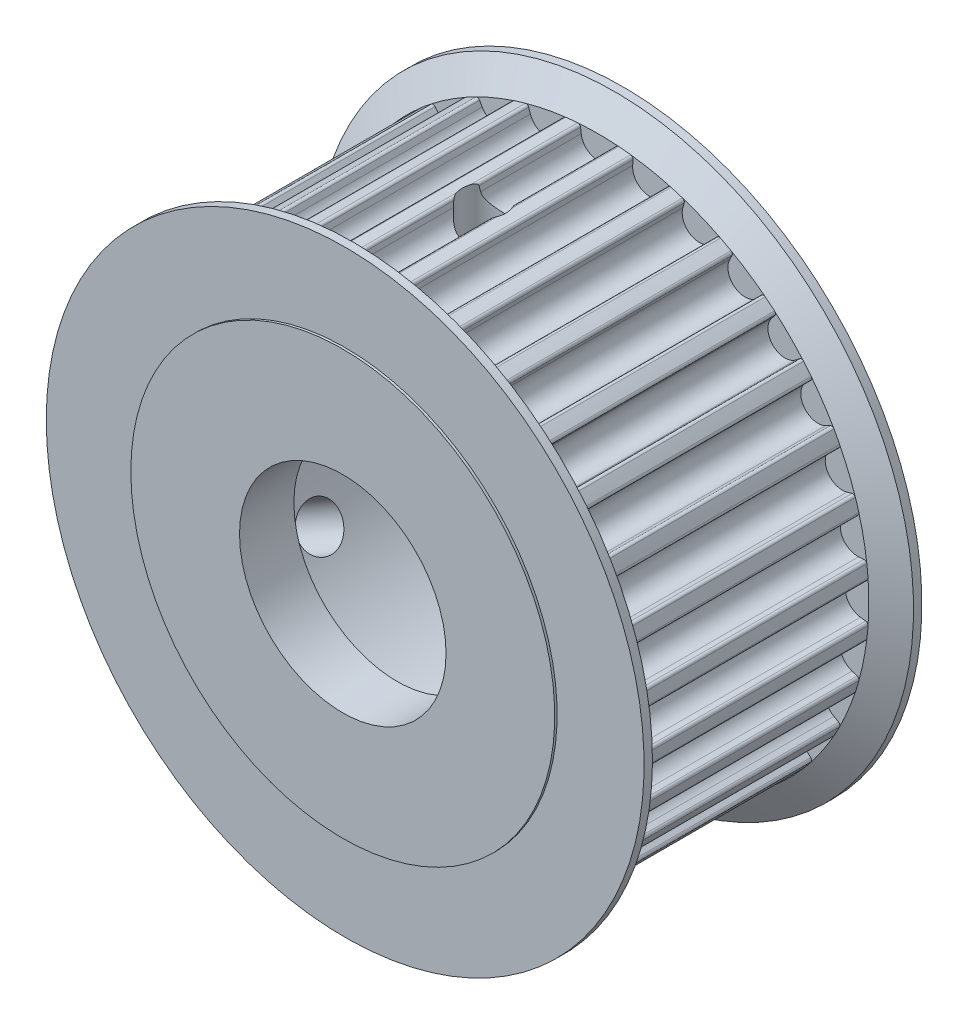
SolidWorks part; units mm, degrees
ref_plane "前视基准面" through (0, 0, 0) normal (0, 0, 1) x (1, 0, 0)
ref_plane "上视基准面" through (0, 0, 0) normal (0, 1, 0) x (1, 0, 0)
ref_plane "右视基准面" through (0, 0, 0) normal (1, 0, 0) x (0, 0, -1)
sketch "草图1" plane through (0, 0, 0) normal (1, 0, 0) x (0, 0, -1)
  line L0 (0, 0) -> (-26, 0) construction
  line L1 (0, 5) -> (-26, 5)
  line L2 (0, 5) -> (0, 19.5)
  line L4 (-0.22, 27.5) -> (-0.99, 27.5)
  line L5 (0, 19.5) -> (-0.22, 19.5)
  line L6 (-2.5, 24.895) -> (-23.5, 24.895)
  line L7 (-0.22, 19.5) -> (-0.22, 27.5)
  line L8 (-0.99, 27.5) -> (-2.5, 24.895)
  line L9 (-13, 0) -> (-13, 25.465) construction
  line L11 (-25.01, 27.5) -> (-23.5, 24.895)
  line L12 (-25.78, 19.5) -> (-25.78, 27.5)
  line L13 (-26, 19.5) -> (-25.78, 19.5)
  line L14 (-25.78, 27.5) -> (-25.01, 27.5)
  line L15 (-26, 5) -> (-26, 19.5)
  point P14 (-13, 5)
  dimension "d" = 10
  dimension "W" = 26
  dimension "K" = 21
  dimension "F" = 55
  dimension "O.D" = 49.79
  dimension "D3" = 25.56
  dimension "D4" = 24.02
  dimension "M" = 39
  dimension "P.D" = 50.93
revolve "旋转1" add sketch "草图1" angle 360 about L0
sketch "草图2" plane through (0, 0, 0) normal (0, 0, 1) x (1, 0, 0)
  line L0 (0, 0) -> (0, 24.895) construction
  line L4 (1.5656, 24.1201) -> (1.625, 24.6042)
  line L5 (-1.5656, 24.1201) -> (-1.625, 24.6042)
  circle A0 centre (0, 0) radius 24.895 construction
  arc A1 (0, 24.895) -> (-1.8921, 24.823) centre (0, 0) ccw construction
  arc A2 (0, 24.895) -> (-1.8921, 24.823) centre (0, 0) ccw construction
  arc A4 (1.8921, 24.823) -> (-1.8921, 24.823) centre (0, 0) ccw
  arc A5 (-1.5656, 24.1201) -> (1.5656, 24.1201) centre (0, 24.3123) ccw
  arc A7 (-1.625, 24.6042) -> (-1.8921, 24.823) centre (-1.8731, 24.5737) ccw
  arc A8 (1.625, 24.6042) -> (1.8921, 24.823) centre (1.8731, 24.5737) cw
  dimension "D2" = 3.25
  dimension "D3" = 7
  dimension "D5" = 0.5
  dimension "D1" = 2.16
extrude "切除-拉伸2" cut sketch "草图2" along normal up to vertex (23.5 mm away) from vertex at 2.5 starting at point (0, 24.895, 2.5)
ref_axis "基准轴1" through (0, 0, -0.625) along (0, 0, 1)
pattern_circular "阵列(圆周)1" count 32 over 360 about axis through (0, 0, 0) along (0, 0, 1) of "切除-拉伸2"
ref_plane "基准面1" through (0, 0, 13) normal (0, 0, 1) x (1, 0, 0)
sketch "草图6" plane through (0, 0, 13) normal (0, 0, 1) x (1, 0, 0)
  line L0 (-2, 27.4272) -> (-2, 4.5826)
  line L1 (0, 5) -> (0, 27.5)
  line L2 (0, 5) -> (0, 27.5) construction
  circle A3 centre (0, 0) radius 5 construction
  arc A4 (0, 5) -> (-2, 4.5826) centre (0, 0) ccw
  circle A7 centre (0, 0) radius 27.5
  arc A8 (0, 27.5) -> (-2, 27.4272) centre (0, 0) ccw
  dimension "D1" = 0
  dimension "Mx" = 4
revolve "切除-旋转1" cut sketch "草图6" angle 360 about L2
cosmetic thread "装饰螺纹线1" parameters "D2"=5.2
pattern_circular "阵列(圆周)2" count 2 over 120 about axis through (0, 0, -0.625) along (0, 0, 1) of "切除-旋转1"
cosmetic thread "装饰螺纹线2" parameters "D2"=5.2
sketch "草图7" plane through (0, 0, 26) normal (0, 0, 1) x (1, 0, 0)
  line L0 (-1.5, 4.7697) -> (-1.5, 6.1697)
  line L1 (-1.5, 6.1697) -> (1.5, 6.1697)
  line L2 (1.5, 6.1697) -> (1.5, 4.7697)
  circle A0 centre (0, 0) radius 5 construction
  arc A1 (1.5, 4.7697) -> (-1.5, 4.7697) centre (0, 0) ccw
  point P0 (0, 6.1697)
  dimension "b" = 3
  dimension "x" = 1.4
extrude "切除-拉伸3" cut sketch "草图7" against normal through all
sketch "草图8" plane through (0, 0, 0) normal (0, 0, -1) x (-1, 0, 0)
  circle A0 centre (0, 0) radius 17.5
  dimension "D1" = 35
extrude "切除-拉伸4" cut sketch "草图8" against normal blind 21
sketch "草图9" plane through (0, 0, 26) normal (0, 0, 1) x (1, 0, 0)
  circle A0 centre (0, 0) radius 9.5
  dimension "D1" = 19
extrude "切除-拉伸5" cut sketch "草图9" against normal blind 21
